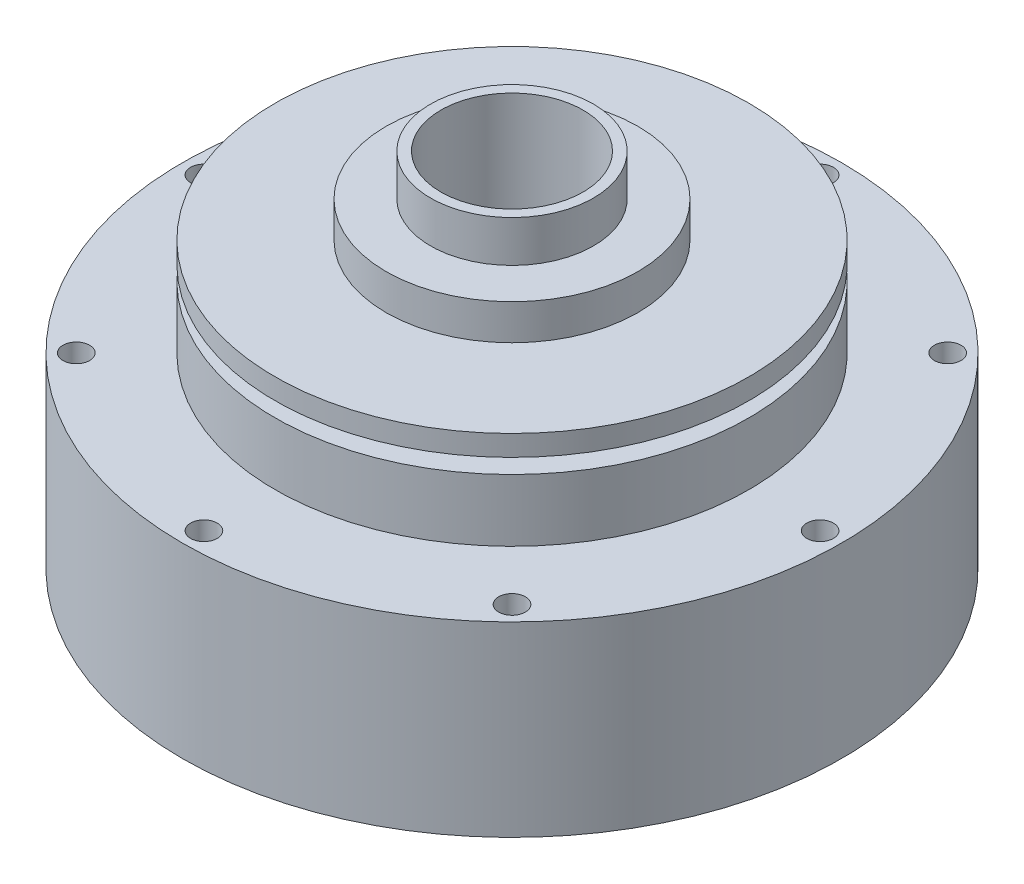
from build123d import *

# Parameters (mm, degrees)
SKETCH_2_R              = 24
CUT_EXTRUDE_1_DEPTH     = 203.193286239
HOLE_WIZARD_M8_1_D      = 9
SKETCH_7_W              = 10
SKETCH_7_H              = 5
HOLE_WIZARD_M10_1_D     = 8.5
HOLE_WIZARD_M10_1_DEPTH = 24.5
HOLE_WIZARD_M10_1_TIP   = 2.553657631


with BuildPart() as part:
    # 草图1 → 旋转1 (revolve)
    with BuildSketch(Plane.XY, mode=Mode.PRIVATE) as revolve_1_sk:
        Polygon((0, 0), (87.5, 0), (87.5, 5), (111.25, 5), (111.25, 68), (80, 68), (80, 101), (42.5, 101), (42.5, 113), (27.5, 113), (27.5, 127), (0, 127), align=None)
    revolve(revolve_1_sk.sketch.rotate(Axis((0, 0, 0), (0, 1, 0)), 90), axis=Axis((0, 0, 0), (0, 1, 0)))

    # 草图2 → 切除-拉伸1 (cut, through all)
    with BuildSketch(Plane(origin=(0, 127, 0), x_dir=(1, 0, 0), z_dir=(0, 1, 0))):
        with Locations(Location((0, 0, 0), (0, 0, 270))):
            Circle(SKETCH_2_R)
    extrude(amount=-CUT_EXTRUDE_1_DEPTH, mode=Mode.SUBTRACT)

    # M8 间隙孔1 (through all)
    with Locations(Plane(origin=(0, 68, 0), x_dir=(1, 0, 0), z_dir=(0, 1, 0))):
        with Locations((0, 104), (73.539105243, 73.539105243), (104, 0), (73.539105243, -73.539105243), (0, -104), (-73.539105243, -73.539105243), (-104, 0), (-73.539105243, 73.539105243)):
            Hole(HOLE_WIZARD_M8_1_D / 2)

    # 草图7 → 切除-旋转1 (revolve, cut)
    with BuildSketch(Plane.XY, mode=Mode.PRIVATE) as cut_revolve_1_sk:
        with Locations((75, 91.5)):
            Rectangle(SKETCH_7_W, SKETCH_7_H)
    revolve(cut_revolve_1_sk.sketch.rotate(Axis((0, 0, 0), (0, 1, 0)), 90), axis=Axis((0, 0, 0), (0, 1, 0)), mode=Mode.SUBTRACT)

    # M10 螺纹孔1
    with Locations(Plane(origin=(0, 0, 0), x_dir=(-1, 0, 0), z_dir=(0, -1, 0))):
        with Locations((0, 67), (47.376154339, 47.376154339), (67, 0), (47.376154339, -47.376154339), (0, -67), (-47.376154339, -47.376154339), (-67, 0), (-47.376154339, 47.376154339)):
            Hole(HOLE_WIZARD_M10_1_D / 2, depth=HOLE_WIZARD_M10_1_DEPTH)
            with Locations((0, 0, -(HOLE_WIZARD_M10_1_DEPTH + HOLE_WIZARD_M10_1_TIP / 2))):  # 118° drill point
                Cone(0, HOLE_WIZARD_M10_1_D / 2, HOLE_WIZARD_M10_1_TIP, mode=Mode.SUBTRACT)


solid = part.part
